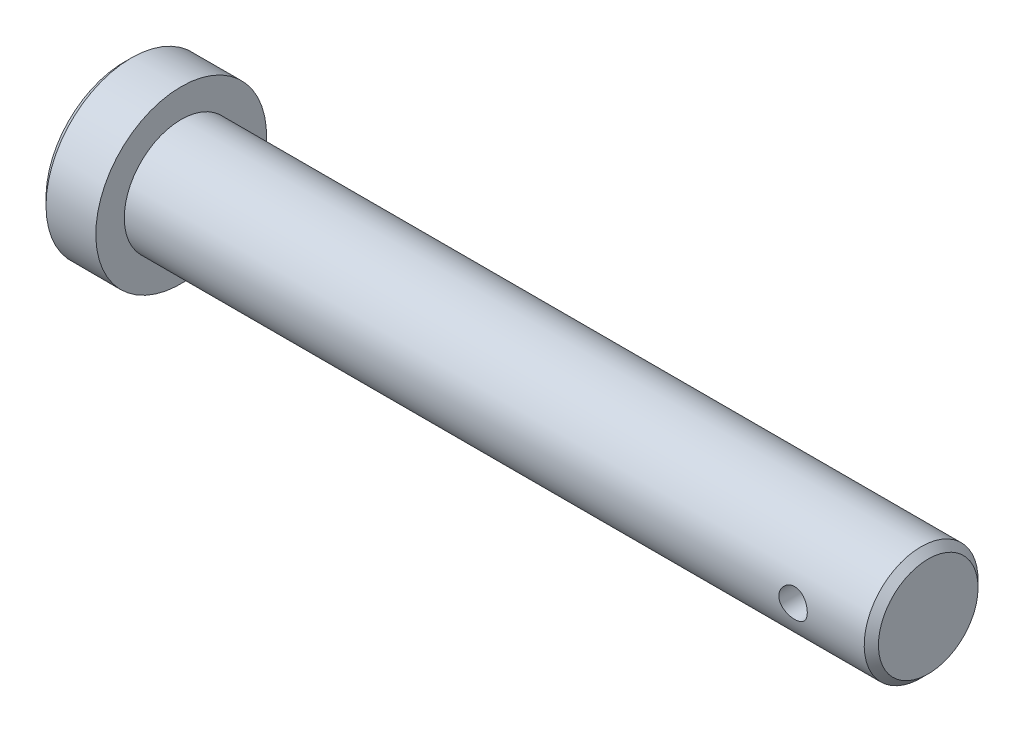
SolidWorks part; units mm, degrees
ref_plane "Front Plane" through (0, 0, 0) normal (0, 0, 1) x (1, 0, 0)
ref_plane "Top Plane" through (0, 0, 0) normal (0, 1, 0) x (1, 0, 0)
ref_plane "Right Plane" through (0, 0, 0) normal (1, 0, 0) x (0, 0, -1)
sketch "Sketch1" plane through (0, 0, 0) normal (0, 0, 1) x (1, 0, 0)
  line L0 (0, 0) -> (-113, 0)
  line L1 (-113, 0) -> (-113, 12)
  line L2 (-113, 12) -> (-105, 12)
  line L3 (-105, 12) -> (-105, 8)
  line L4 (-105, 8) -> (0, 8)
  line L5 (0, 8) -> (0, 0)
  dimension "D1" = 8
  dimension "D2" = 12
  dimension "D3" = 8
  dimension "D4" = 105
revolve "Revolve1" add sketch "Sketch1" angle 360 about L0
sketch "Sketch2" plane through (0, 0, 0) normal (0, 0, 1) x (1, 0, 0)
  line L0 (-105, -12) -> (-105, 12) construction
  circle A0 centre (-11, 0) radius 2
  dimension "D1" = 4
  dimension "D2" = 94
extrude "Cut-Extrude1" cut sketch "Sketch2" against normal through all both and the other way through all
chamfer "Chamfer1" distance 1 angle 45 1 edges at (0, 8, 0)
chamfer "Chamfer2" distance 1 angle 45 1 edges at (-113, 12, 0)
